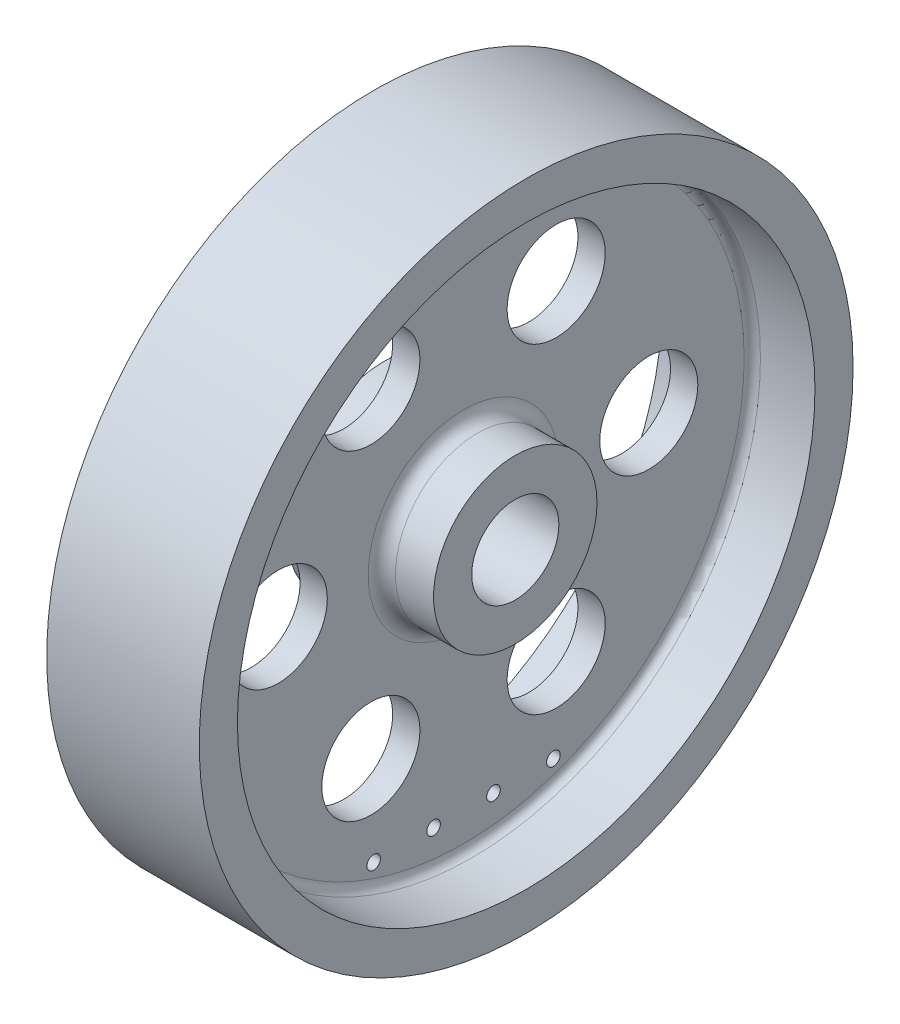
SolidWorks part; units mm, degrees
material "灰铸铁 HT200 "
ref_plane "Front Plane" through (0, 0, 0) normal (0, 0, 1) x (1, 0, 0)
ref_plane "Top Plane" through (0, 0, 0) normal (0, 1, 0) x (1, 0, 0)
ref_plane "Right Plane" through (0, 0, 0) normal (1, 0, 0) x (0, 0, -1)
sketch "Sketch2" plane through (0, 0, 0) normal (0, 0, 1) x (1, 0, 0)
  line L0 (225.6571, 0) -> (0, 0) construction
  line L1 (-20, 600) -> (-20, 530)
  line L2 (260, 600) -> (260, 530)
  line L3 (95, 515) -> (95, 205)
  line L4 (145, 515) -> (145, 175)
  line L5 (0, 180) -> (0, 105)
  line L6 (240, 150) -> (240, 80)
  line L7 (70, 180) -> (0, 180)
  line L8 (170, 150) -> (240, 150)
  line L9 (260, 530) -> (160, 530)
  line L10 (80, 530) -> (-20, 530)
  line L11 (0, 105) -> (70, 105)
  line L12 (70, 105) -> (70, 80)
  line L13 (70, 80) -> (240, 80)
  line L14 (-20, 600) -> (260, 600)
  line L15 (120, 324.3302) -> (120, 85.9832) construction
  arc A0 (145, 175) -> (170, 150) centre (170, 175) ccw
  arc A4 (70, 180) -> (95, 205) centre (70, 205) ccw
  arc A6 (160, 530) -> (145, 515) centre (160, 515) ccw
  arc A7 (95, 515) -> (80, 530) centre (80, 515) ccw
  dimension "D9" = 25
  dimension "D10" = 25
  dimension "D11" = 15
  dimension "D13" = 15
  dimension "D1" = 80
  dimension "D2" = 105
  dimension "D3" = 70
  dimension "D4" = 240
  dimension "D5" = 180
  dimension "D6" = 150
  dimension "D7" = 20
  dimension "D8" = 50
  dimension "D12" = 530
  dimension "D14" = 600
  dimension "D15" = 280
sketch "Sketch3" plane through (538.8474, 0, 0) normal (1, 0, 0) x (0, 0, -1)
  line L0 (0, -1.8755) -> (826.9212, -1.8755) construction
  line L1 (-826.9212, -1.8755) -> (-85, -1.8755) construction
  line L2 (0, 803.1837) -> (0, -867.453) construction
  line L3 (-165.556, 284.8759) -> (-284.8898, 491.5681) construction
  line L4 (-165.556, -288.627) -> (-284.8898, -495.3192) construction
  line L5 (165.556, 284.8759) -> (284.8898, 491.5681) construction
  line L6 (165.556, -288.627) -> (284.8898, -495.3192) construction
  line L7 (-240.2543, 578.1245) -> (242.1135, 578.1245) construction
  line L8 (-60, 620.3139) -> (-60, 535.9351) construction
  line L9 (-180, 621.6856) -> (-180, 534.5633) construction
  line L10 (180, 621.6856) -> (180, 534.5633) construction
  line L11 (60, 620.3139) -> (60, 535.9351) construction
  line L12 (106.8046, 59.7882) -> (151.3767, 85.5219) construction
  line L13 (-103.4525, 57.8528) -> (-149.6234, 84.5096) construction
  line L14 (0, 93.1245) -> (-1, 83.1186)
  line L15 (0, 93.1245) -> (1, 83.1186)
  circle A0 centre (0, 0) radius 450 construction
  circle A1 centre (0, 0) radius 757.5
  circle A2 centre (0, -1.8755) radius 677.5
  circle A3 centre (0, -1.8755) radius 210
  circle A4 centre (0, -1.8755) radius 112.5
  arc A5 (-1, 83.1186) -> (1, 83.1186) centre (0, -1.8755) ccw
  circle A6 centre (-449.9961, -1.8755) radius 60
  circle A7 centre (-224.998, -391.5836) radius 60
  circle A8 centre (224.998, -391.5836) radius 60
  circle A9 centre (449.9961, -1.8755) radius 60
  circle A10 centre (224.998, 387.8325) radius 60
  circle A11 centre (-224.998, 387.8325) radius 60
  circle A12 centre (-180, 578.1245) radius 12.5
  circle A13 centre (-60, 578.1245) radius 12.5
  circle A14 centre (60, 578.1245) radius 12.5
  circle A15 centre (180, 578.1245) radius 12.5
  circle A16 centre (0, -1.8755) radius 145 construction
  circle A17 centre (0, -146.8755) radius 10
  arc A18 (12.9869, -146.2928) -> (0, -159.8755) centre (0, -146.8755) ccw
  arc A19 (131.5625, 59.0861) -> (114.3154, 64.1245) centre (125.5737, 70.6245) ccw
  circle A20 centre (125.5737, 70.6245) radius 10
  arc A21 (-114.3154, 64.1245) -> (-131.5625, 59.0861) centre (-125.5737, 70.6245) ccw
  circle A22 centre (-125.5737, 70.6245) radius 10
revolve "Revolve1" add sketch "Sketch2" angle 360 about L0
sketch "Sketch4" plane through (0, 0, 0) normal (1, 0, 0) x (0, 0, -1)
  line L0 (0, 0) -> (0, 216.8731) construction
  line L1 (0, 0) -> (-210.0698, 363.8516) construction
  circle A0 centre (0, 0) radius 340 construction
  circle A1 centre (-170, 294.4486) radius 90
  dimension "D1" = 680
  dimension "D2" = 180
  dimension "D3" = 30
extrude "Cut-Extrude1" cut sketch "Sketch4" along normal blind 343
pattern_circular "CirPattern1" count 6 over 360 about axis through (0, 0, 0) along (1, 0, 0) of "Cut-Extrude1"
sketch "Sketch5" plane through (0, 0, 0) normal (-1, 0, 0) x (0, 0, 1)
  line L0 (0, 0) -> (66.25, 0) construction
  line L1 (0, 0) -> (66.25, 114.7484) construction
  dimension "D1" = 60
  dimension "D2" = 132.5
hole_wizard "M24 Tapped Hole1" positions "3DSketch1" profile "Sketch6" tap size "M24" standard "GB"
sketch3d "3DSketch1"
  point P0 (0, 114.7484, 66.25)
sketch "Sketch6" plane through (0, 114.7484, 66.25) normal (0, 1, 0) x (0, 0, 1)
  line L0 (0, 0) -> (0, 46.309)
  line L1 (0, 46.309) -> (10.5, 40)
  line L2 (10.5, 40) -> (10.5, 0)
  line L5 (10.5, 0) -> (0, 0)
  line L10 (0, 46.309) -> (-10.5, 40) construction
  line L11 (0, -6.35) -> (0, 107.95) construction
  dimension "螺纹孔钻头直径" = 21
  dimension "螺纹孔钻头深度" = 40
  dimension "导头角度" = 118
cosmetic thread "hole cosmetic thread 1" parameters "D1"=40, "D2"=24
pattern_circular "CirPattern2" count 3 over 360 about axis through (0, 0, 0) along (1, 0, 0) of "M24 Tapped Hole1"
sketch "Sketch8" plane through (0, 0, 0) normal (1, 0, 0) x (0, 0, -1)
  line L0 (0, 0) -> (0, -462) construction
  line L1 (165, -462) -> (-165, -462) construction
  circle A0 centre (-55, -462) radius 12.5
  circle A1 centre (-165, -462) radius 12.5
  circle A2 centre (55, -462) radius 12.5
  circle A3 centre (165, -462) radius 12.5
  point P6 (0, -462)
  dimension "D2" = 25
  dimension "D3" = 110
  dimension "D1" = 462
  dimension "D4" = 55
extrude "Cut-Extrude3" cut sketch "Sketch8" along normal blind 238
